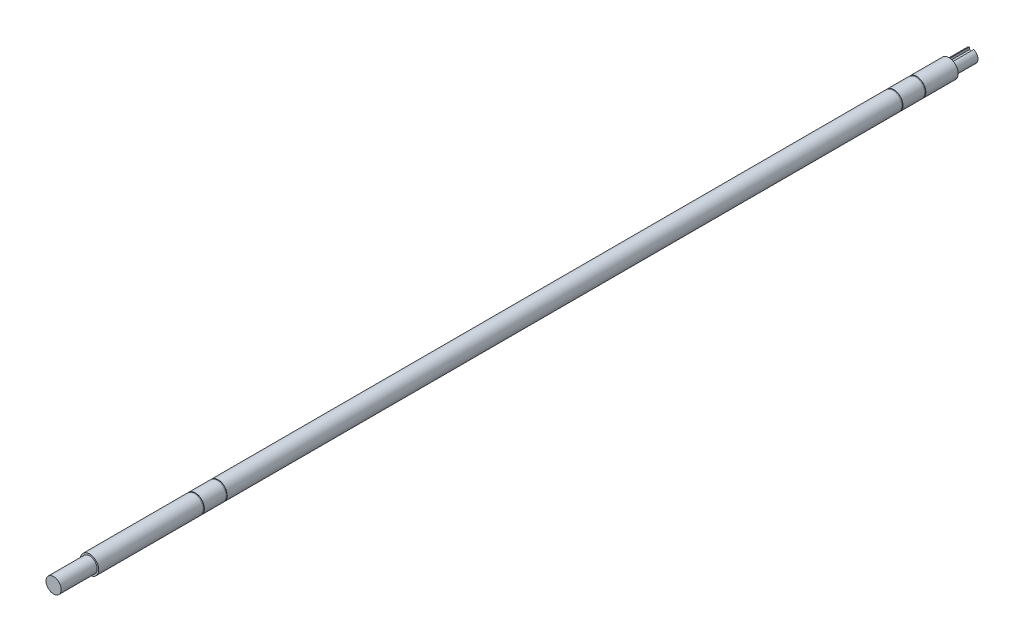
from build123d import *

# Parameters (mm, degrees)
SKETCH_1_R               = 7
EXTRUDE_1_DEPTH          = 450
SKETCH_2_R               = 8.5
EXTRUDE_2_DEPTH          = 416.8
CUT_EXTRUDE_START        = -33.2
SKETCH_3_R               = 8.5
SKETCH_3_R_2             = 6
CUT_EXTRUDE_1_DEPTH      = 33.2
CUT_EXTRUDE_2_DEPTH      = 451.160526923
CUT_EXTRUDE_2_DEPTH_BACK = 451.160526923
SKETCH_4_W               = 12
SKETCH_4_H               = 12.45
MOVE_FACE_1_BY           = 40
MOVE_FACE_1_2_BY         = 40
CUT_EXTRUDE_11_DEPTH     = 2.5
HOLE_WIZARD_M4_1_D       = 3.3
HOLE_WIZARD_M4_1_DEPTH   = 10.1
HOLE_WIZARD_M4_1_TIP     = 0.991420021
CUT_EXTRUDE_START_2      = 1.1
SKETCH_35_R              = 8.5
SKETCH_35_R_2            = 8.1
CUT_EXTRUDE_12_DEPTH     = 1.1
SKETCH_36_R              = 8.5
SKETCH_36_R_2            = 8.1
CUT_EXTRUDE_13_DEPTH     = 1.1
SKETCH_37_R              = 8.5
SKETCH_37_R_2            = 8.1
CUT_EXTRUDE_14_DEPTH     = 1.1
SKETCH_38_R              = 8.5
SKETCH_38_R_2            = 8.1
CUT_EXTRUDE_15_DEPTH     = 1.1


with BuildPart() as part:
    # 草图1 → 凸台-拉伸1 (new, symmetric)
    with BuildSketch(Plane.XY):
        Circle(SKETCH_1_R)
    extrude(amount=EXTRUDE_1_DEPTH, both=True)

    # 草图2 → 凸台-拉伸2 (add, symmetric)
    with BuildSketch(Plane.XY):
        Circle(SKETCH_2_R)
    extrude(amount=EXTRUDE_2_DEPTH, both=True)

    # 草图3 → 切除-拉伸1 (cut)
    with BuildSketch(Plane(origin=(0, 0, -450), x_dir=(-1, 0, 0), z_dir=(0, 0, -1)).offset(CUT_EXTRUDE_START)):
        with Locations(Location((0, 0, 0), (0, 0, 180))):
            Circle(SKETCH_3_R)
        Circle(SKETCH_3_R_2, mode=Mode.SUBTRACT)
    extrude(amount=CUT_EXTRUDE_1_DEPTH, mode=Mode.SUBTRACT)

    # 草图4 → 切除-拉伸2 (cut, two sides: drawn at the far end of the back side and taken through both)
    with BuildSketch(Plane(origin=(0, 0, 0), x_dir=(1, 0, 0), z_dir=(0, 1, 0)).offset(-CUT_EXTRUDE_2_DEPTH_BACK)):
        with Locations((0, 443.775)):
            Rectangle(SKETCH_4_W, SKETCH_4_H)
    extrude(amount=CUT_EXTRUDE_2_DEPTH + CUT_EXTRUDE_2_DEPTH_BACK, mode=Mode.SUBTRACT)

    # Move Face 1: a face moved inward by 40.0
    extrude(part.faces().sort_by_distance((0, 0, -437.55))[0], amount=MOVE_FACE_1_BY, dir=(0, 0, 1), mode=Mode.SUBTRACT)

    # Move Face 1 2: a face moved inward by 40.0
    extrude(part.faces().sort_by_distance((0, -6.8, -416.8))[0], amount=MOVE_FACE_1_2_BY, dir=(0, 0, 1), mode=Mode.SUBTRACT)

    # 草图31 → 切除-拉伸11 (cut)
    with BuildSketch(Plane(origin=(0, 6, -397.55), x_dir=(0, 0, 1), z_dir=(0, 1, 0))):
        with BuildLine():
            Line((-1, 2), (17.75, 2))
            ThreePointArc((17.75, 2), (19.75, 0), (17.75, -2))
            Line((17.75, -2), (-1, -2))
            ThreePointArc((-1, -2), (-3, 0), (-1, 2))
        make_face()
    extrude(amount=-CUT_EXTRUDE_11_DEPTH, mode=Mode.SUBTRACT)

    # M4 螺纹孔1
    with Locations(Plane(origin=(0, 0, -397.55), x_dir=(-1, 0, 0), z_dir=(0, 0, -1))):
        with Locations((0, 0)):
            Hole(HOLE_WIZARD_M4_1_D / 2, depth=HOLE_WIZARD_M4_1_DEPTH)
            with Locations((0, 0, -(HOLE_WIZARD_M4_1_DEPTH + HOLE_WIZARD_M4_1_TIP / 2))):  # 118° drill point
                Cone(0, HOLE_WIZARD_M4_1_D / 2, HOLE_WIZARD_M4_1_TIP, mode=Mode.SUBTRACT)

    # 草图35 → 切除-拉伸12 (cut)
    with BuildSketch(Plane.XY.offset(319.2).offset(CUT_EXTRUDE_START_2)):
        Circle(SKETCH_35_R)
        Circle(SKETCH_35_R_2, mode=Mode.SUBTRACT)
    extrude(amount=-CUT_EXTRUDE_12_DEPTH, mode=Mode.SUBTRACT)

    # 草图36 → 切除-拉伸13 (cut)
    with BuildSketch(Plane.XY.offset(298.1).offset(CUT_EXTRUDE_START_2)):
        Circle(SKETCH_36_R)
        Circle(SKETCH_36_R_2, mode=Mode.SUBTRACT)
    extrude(amount=-CUT_EXTRUDE_13_DEPTH, mode=Mode.SUBTRACT)

    # 草图37 → 切除-拉伸14 (cut)
    with BuildSketch(Plane.XY.offset(-325.8).offset(CUT_EXTRUDE_START_2)):
        Circle(SKETCH_37_R)
        Circle(SKETCH_37_R_2, mode=Mode.SUBTRACT)
    extrude(amount=-CUT_EXTRUDE_14_DEPTH, mode=Mode.SUBTRACT)

    # 草图38 → 切除-拉伸15 (cut)
    with BuildSketch(Plane.XY.offset(-346.9).offset(CUT_EXTRUDE_START_2)):
        Circle(SKETCH_38_R)
        Circle(SKETCH_38_R_2, mode=Mode.SUBTRACT)
    extrude(amount=-CUT_EXTRUDE_15_DEPTH, mode=Mode.SUBTRACT)


solid = part.part
